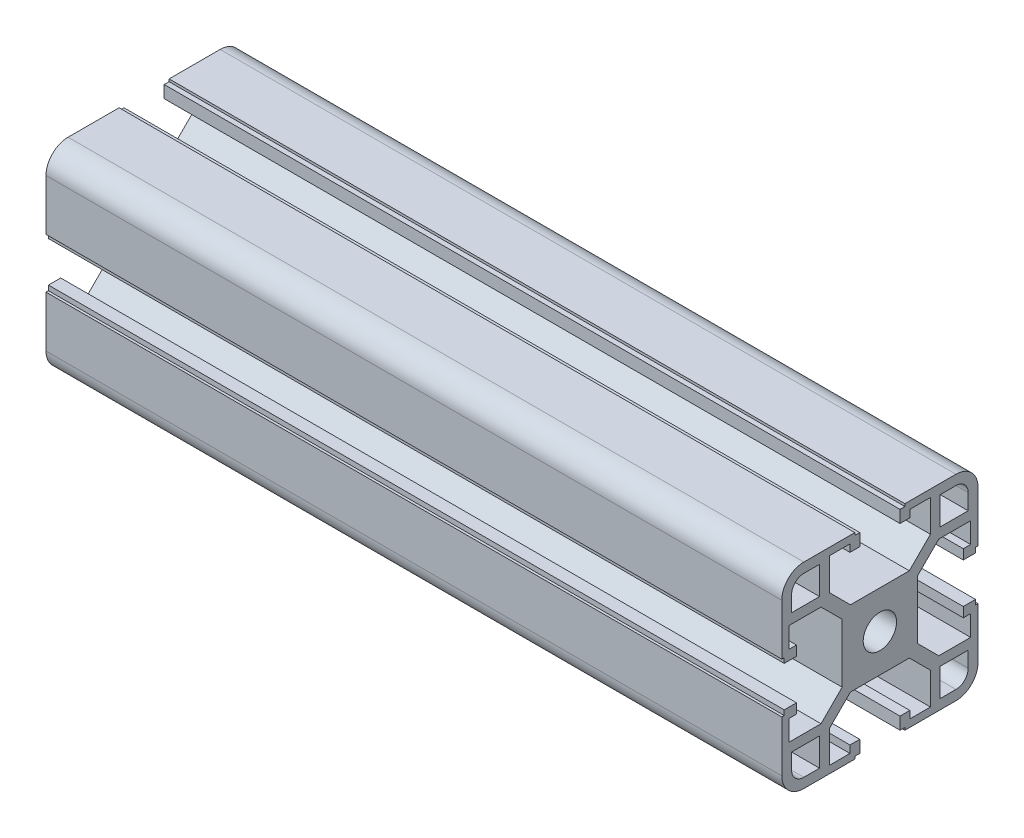
SolidWorks part; units mm, degrees
ref_plane "Front Plane" through (0, 0, 0) normal (0, 0, 1) x (1, 0, 0)
ref_plane "Top Plane" through (0, 0, 0) normal (0, 1, 0) x (1, 0, 0)
ref_plane "Right Plane" through (0, 0, 0) normal (1, 0, 0) x (0, 0, -1)
sketch "草图1" plane through (0, 0, 0) normal (0, 0, 1) x (1, 0, 0)
  line L0 (-984.975, 0) -> (-834.975, 0)
  dimension "D1" = 150
other "Aluminium profile 40 X 40B X R4.5(1)"
ref_plane "Plane1" through (-984.975, 0, 0) normal (1, 0, 0) x (0, 1, 0)
sketch "Sketch1" plane through (-984.975, 0, 0) normal (1, 0, 0) x (0, 1, 0)
  line L0 (-5.1, 20) -> (-5.1, 19.5)
  line L1 (-5.1, 19.5) -> (-4.1, 19.5)
  line L2 (-4.1, 19.5) -> (-4.1, 17)
  line L3 (-6.1, 18.5) -> (-10.3, 18.5)
  line L4 (-15.5, -20) -> (-5.1, -20)
  line L5 (-20, -15.5) -> (-20, -5.1)
  line L6 (15.5, 20) -> (5.1, 20)
  line L7 (20, 15.5) -> (20, 5.1)
  line L8 (0, 14.8756) -> (0, 0) construction
  line L9 (0, 0) -> (14.1675, 0) construction
  line L10 (-10.3, 18.5) -> (-10.3, 12)
  line L11 (-10.3, 12) -> (-6, 7.7)
  line L12 (-6, 7.7) -> (6, 7.7)
  line L13 (10.3, 12) -> (6, 7.7)
  line L14 (10.3, 18.5) -> (10.3, 12)
  line L15 (6.1, 18.5) -> (10.3, 18.5)
  line L16 (4.1, 19.5) -> (4.1, 17)
  line L17 (5.1, 19.5) -> (4.1, 19.5)
  line L18 (5.1, 20) -> (5.1, 19.5)
  line L19 (-5.1, 20) -> (-15.5, 20)
  line L20 (20, 5.1) -> (19.5, 5.1)
  line L21 (12.3, 18) -> (15.5, 18)
  line L22 (12.3, 18) -> (12.3, 12.3)
  line L23 (12.3, 12.3) -> (18, 12.3)
  line L24 (18, 15.5) -> (18, 12.3)
  line L25 (19.5, 5.1) -> (19.5, 4.1)
  line L26 (19.5, 4.1) -> (17, 4.1)
  line L27 (17, 6.1) -> (17, 4.1)
  line L28 (18.5, 6.1) -> (17, 6.1)
  line L29 (18.5, 6.1) -> (18.5, 10.3)
  line L30 (18.5, 10.3) -> (12, 10.3)
  line L31 (12, 10.3) -> (7.7, 6)
  line L32 (7.7, 6) -> (7.7, -6)
  line L33 (12, -10.3) -> (7.7, -6)
  line L34 (18.5, -10.3) -> (12, -10.3)
  line L35 (18.5, -6.1) -> (18.5, -10.3)
  line L36 (18.5, -6.1) -> (17, -6.1)
  line L37 (17, -4.1) -> (17, -6.1)
  line L38 (19.5, -4.1) -> (17, -4.1)
  line L39 (19.5, -5.1) -> (19.5, -4.1)
  line L40 (20, -5.1) -> (19.5, -5.1)
  line L41 (5.1, -20) -> (5.1, -19.5)
  line L42 (5.1, -19.5) -> (4.1, -19.5)
  line L43 (4.1, -19.5) -> (4.1, -17)
  line L44 (6.1, -17) -> (4.1, -17)
  line L45 (6.1, -18.5) -> (6.1, -17)
  line L46 (6.1, -18.5) -> (10.3, -18.5)
  line L47 (10.3, -18.5) -> (10.3, -12)
  line L48 (10.3, -12) -> (6, -7.7)
  line L49 (6, -7.7) -> (-6, -7.7)
  line L50 (-10.3, -12) -> (-6, -7.7)
  line L51 (-10.3, -18.5) -> (-10.3, -12)
  line L52 (-6.1, -18.5) -> (-10.3, -18.5)
  line L53 (-6.1, -18.5) -> (-6.1, -17)
  line L54 (-4.1, -17) -> (-6.1, -17)
  line L55 (-4.1, -19.5) -> (-4.1, -17)
  line L56 (-5.1, -19.5) -> (-4.1, -19.5)
  line L57 (-5.1, -20) -> (-5.1, -19.5)
  line L58 (-20, -5.1) -> (-19.5, -5.1)
  line L59 (5.1, -20) -> (15.5, -20)
  line L60 (-20, 5.1) -> (-20, 15.5)
  line L61 (-19.5, -5.1) -> (-19.5, -4.1)
  line L62 (-6.1, 18.5) -> (-6.1, 17)
  line L63 (-6.1, 17) -> (-4.1, 17)
  line L64 (6.1, 18.5) -> (6.1, 17)
  line L65 (4.1, 17) -> (6.1, 17)
  line L66 (-19.5, -4.1) -> (-17, -4.1)
  line L67 (-15.5, 18) -> (-12.3, 18)
  line L68 (-18, 15.5) -> (-18, 12.3)
  line L69 (-18, 12.3) -> (-12.3, 12.3)
  line L70 (-12.3, 18) -> (-12.3, 12.3)
  line L71 (-17, -6.1) -> (-17, -4.1)
  line L72 (-18.5, -6.1) -> (-17, -6.1)
  line L73 (-18.5, -6.1) -> (-18.5, -10.3)
  line L74 (-18.5, -10.3) -> (-12, -10.3)
  line L75 (-12, -10.3) -> (-7.7, -6)
  line L76 (-7.7, -6) -> (-7.7, 6)
  line L77 (-12, 10.3) -> (-7.7, 6)
  line L78 (-18.5, 10.3) -> (-12, 10.3)
  line L79 (-18.5, 6.1) -> (-18.5, 10.3)
  line L80 (-18.5, 6.1) -> (-17, 6.1)
  line L81 (-17, 4.1) -> (-17, 6.1)
  line L82 (-19.5, 4.1) -> (-17, 4.1)
  line L83 (-19.5, 5.1) -> (-19.5, 4.1)
  line L84 (-20, 5.1) -> (-19.5, 5.1)
  line L85 (20, -5.1) -> (20, -15.5)
  line L87 (-18, -12.3) -> (-12.3, -12.3)
  line L88 (-18, -12.3) -> (-18, -15.5)
  line L89 (-15.5, -18) -> (-12.3, -18)
  line L90 (-12.3, -12.3) -> (-12.3, -18)
  line L91 (12.3, -12.3) -> (18, -12.3)
  line L92 (12.3, -12.3) -> (12.3, -18)
  line L93 (12.3, -18) -> (15.5, -18)
  line L94 (18, -12.3) -> (18, -15.5)
  circle A0 centre (0, 0) radius 3.4
  arc A1 (-20, 15.5) -> (-15.5, 20) centre (-15.5, 15.5) cw
  arc A2 (20, 15.5) -> (15.5, 20) centre (15.5, 15.5) ccw
  arc A3 (-15.5, -20) -> (-20, -15.5) centre (-15.5, -15.5) cw
  arc A4 (15.5, -20) -> (20, -15.5) centre (15.5, -15.5) ccw
  arc A5 (-15.5, 18) -> (-18, 15.5) centre (-15.5, 15.5) ccw
  arc A6 (18, 15.5) -> (15.5, 18) centre (15.5, 15.5) ccw
  arc A7 (18, -15.5) -> (15.5, -18) centre (15.5, -15.5) cw
  arc A8 (-18, -15.5) -> (-15.5, -18) centre (-15.5, -15.5) ccw
  point P2 (0, 10)
  point P4 (0, 0)
  point P5 (-20, -20)
  point P6 (20, -20)
  point P7 (20, 20)
  point P8 (-20, 20)
  point P36 (-20, 20)
  point P39 (20, 20)
  point P121 (0, 0)
  dimension "D1" = 20.6
  dimension "D2" = 40
  dimension "D3" = 8.2
  dimension "D4" = 10.2
  dimension "D5" = 12.3
  dimension "D6" = 6.8
  dimension "D7" = 4.5
  dimension "D8" = 45
  dimension "D12" = 2
  dimension "D13" = 5.7
  dimension "D14" = 2
  dimension "D18" = 2.5
  dimension "D19" = 2.5
  dimension "D15" = 2.5
  dimension "D9" = 0.5
  dimension "D10" = 1.5
  dimension "D11" = 12
  dimension "D16" = 3
  dimension "D17" = 2
  dimension "D20" = 2
  dimension "D21" = 2
